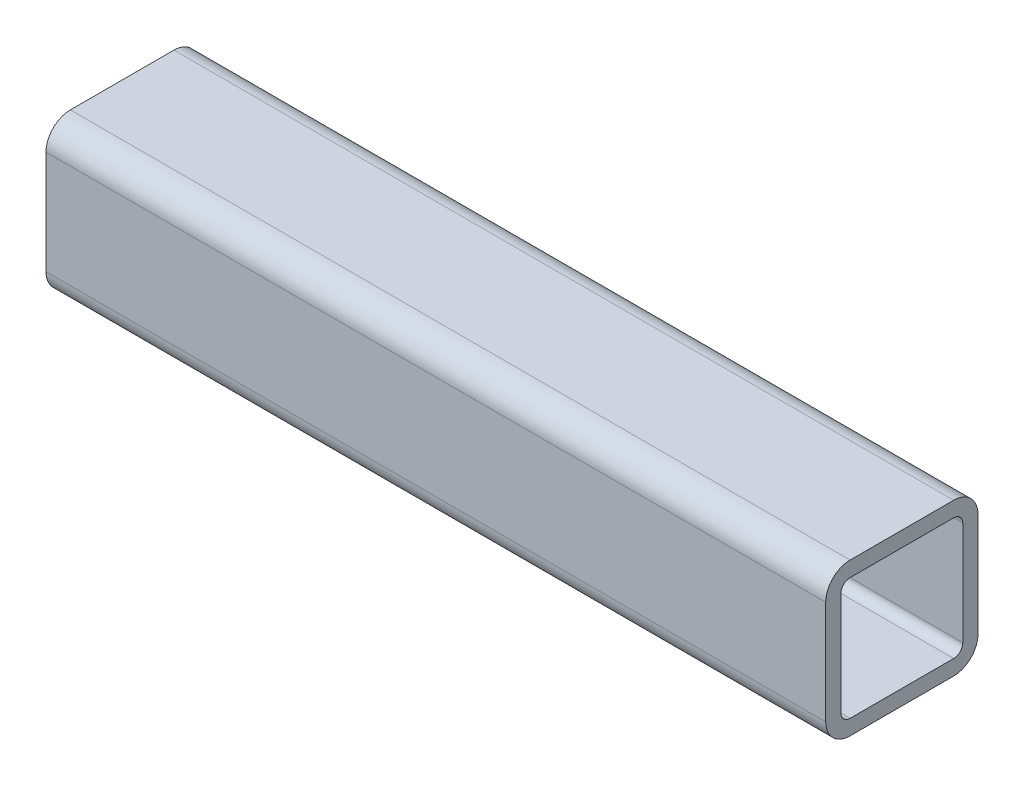
SolidWorks part; units mm, degrees
ref_plane "Front Plane" through (0, 0, 0) normal (0, 0, 1) x (1, 0, 0)
ref_plane "Top Plane" through (0, 0, 0) normal (0, 1, 0) x (1, 0, 0)
ref_plane "Right Plane" through (0, 0, 0) normal (1, 0, 0) x (0, 0, -1)
sketch "草图1" plane through (0, 0, 0) normal (0, 0, 1) x (1, 0, 0)
  line L0 (-88.4341, 0) -> (167.5659, 0)
  dimension "D1" = 256
other "Cold-formed square hollow section GB/T 6728-2002 50 X 50 X 4(1)"
ref_plane "Plane1" through (-88.4341, 0, 0) normal (1, 0, 0) x (0, 1, 0)
sketch "Sketch1" plane through (-88.4341, 0, 0) normal (1, 0, 0) x (0, 1, 0)
  line L0 (-17, -20) -> (17, -20)
  line L1 (-20, -17) -> (-20, 17)
  line L2 (17, 20) -> (-17, 20)
  line L3 (20, 17) -> (20, -17)
  line L4 (-17, -25) -> (17, -25)
  line L5 (-25, -17) -> (-25, 17)
  line L6 (17, 25) -> (-17, 25)
  line L7 (25, 17) -> (25, -17)
  arc A0 (25, 17) -> (17, 25) centre (17, 17) ccw
  arc A1 (17, -25) -> (25, -17) centre (17, -17) ccw
  arc A2 (-25, -17) -> (-17, -25) centre (-17, -17) ccw
  arc A3 (-17, 25) -> (-25, 17) centre (-17, 17) ccw
  arc A4 (-17, 20) -> (-20, 17) centre (-17, 17) ccw
  arc A5 (20, 17) -> (17, 20) centre (17, 17) ccw
  arc A6 (17, -20) -> (20, -17) centre (17, -17) ccw
  arc A7 (-20, -17) -> (-17, -20) centre (-17, -17) ccw
  point P0 (-25, 0)
  point P1 (25, 0)
  point P2 (0, 25)
  point P3 (0, -25)
  point P4 (0, 0)
  point P5 (-25, -25)
  point P6 (25, -25)
  point P7 (25, 25)
  point P8 (-25, 25)
  point P33 (0, 0)
  dimension "D1" = 8
  dimension "Thickness" = 5
  dimension "V_leg" = 50
